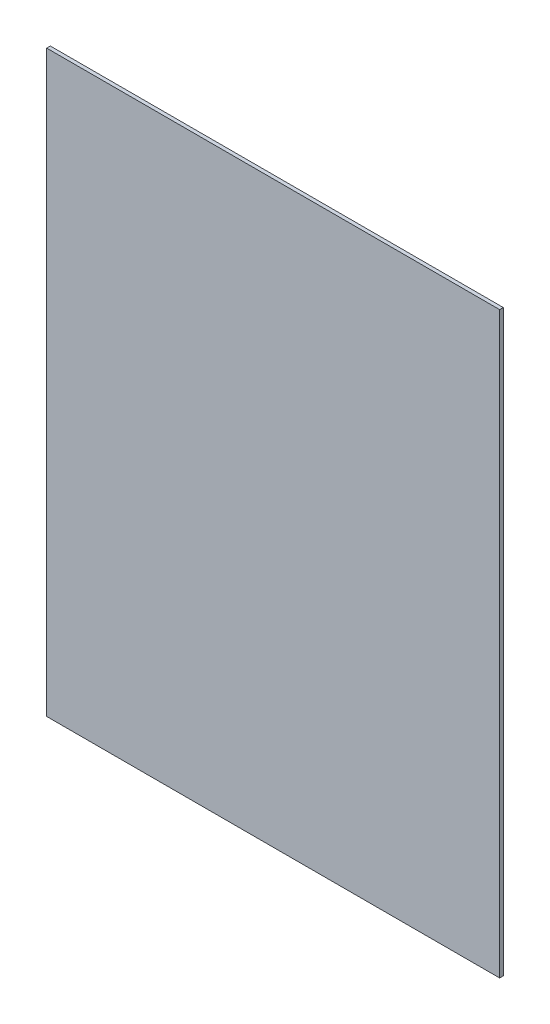
SolidWorks part; units mm, degrees
material "PMMA(有机玻璃)"
ref_plane "前视" through (0, 0, 0) normal (0, 0, 1) x (1, 0, 0)
ref_plane "上视" through (0, 0, 0) normal (0, 1, 0) x (1, 0, 0)
ref_plane "右视" through (0, 0, 0) normal (1, 0, 0) x (0, 0, -1)
sketch "草图1" plane through (0, 0, 0) normal (0, 0, 1) x (1, 0, 0)
  line L1 (-309.5, 395.5) -> (309.5, 395.5)
  line L2 (-309.5, 395.5) -> (-309.5, -395.5)
  line L3 (-309.5, -395.5) -> (309.5, -395.5)
  line L4 (309.5, 395.5) -> (309.5, -395.5)
  line L5 (-309.5, 395.5) -> (309.5, -395.5) construction
  line L6 (-309.5, -395.5) -> (309.5, 395.5) construction
  point P0 (0, 0)
  dimension "D1" = 791
  dimension "D2" = 619
extrude "凸台-拉伸1" add sketch "草图1" along normal blind 5
